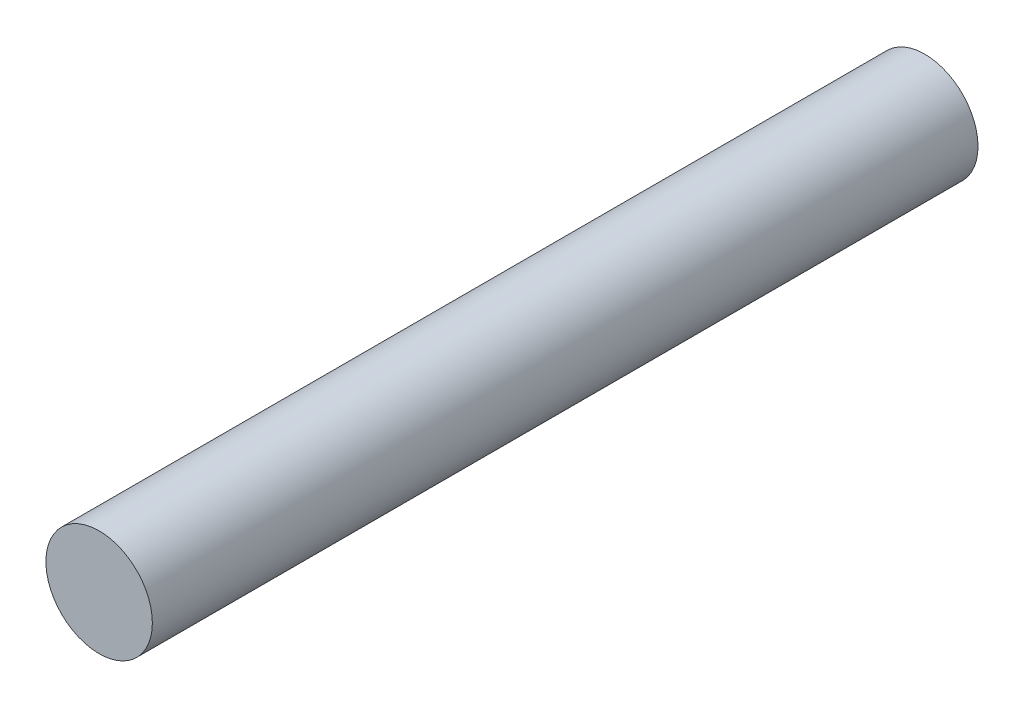
from build123d import *

# Parameters (mm, degrees)
SKETCH_1_R      = 2.45
EXTRUDE_1_DEPTH = 38


with BuildPart() as part:
    # 草图1 → 凸台-拉伸1 (new body)
    with BuildSketch(Plane.XY):
        Circle(SKETCH_1_R)
    extrude(amount=EXTRUDE_1_DEPTH)


solid = part.part
